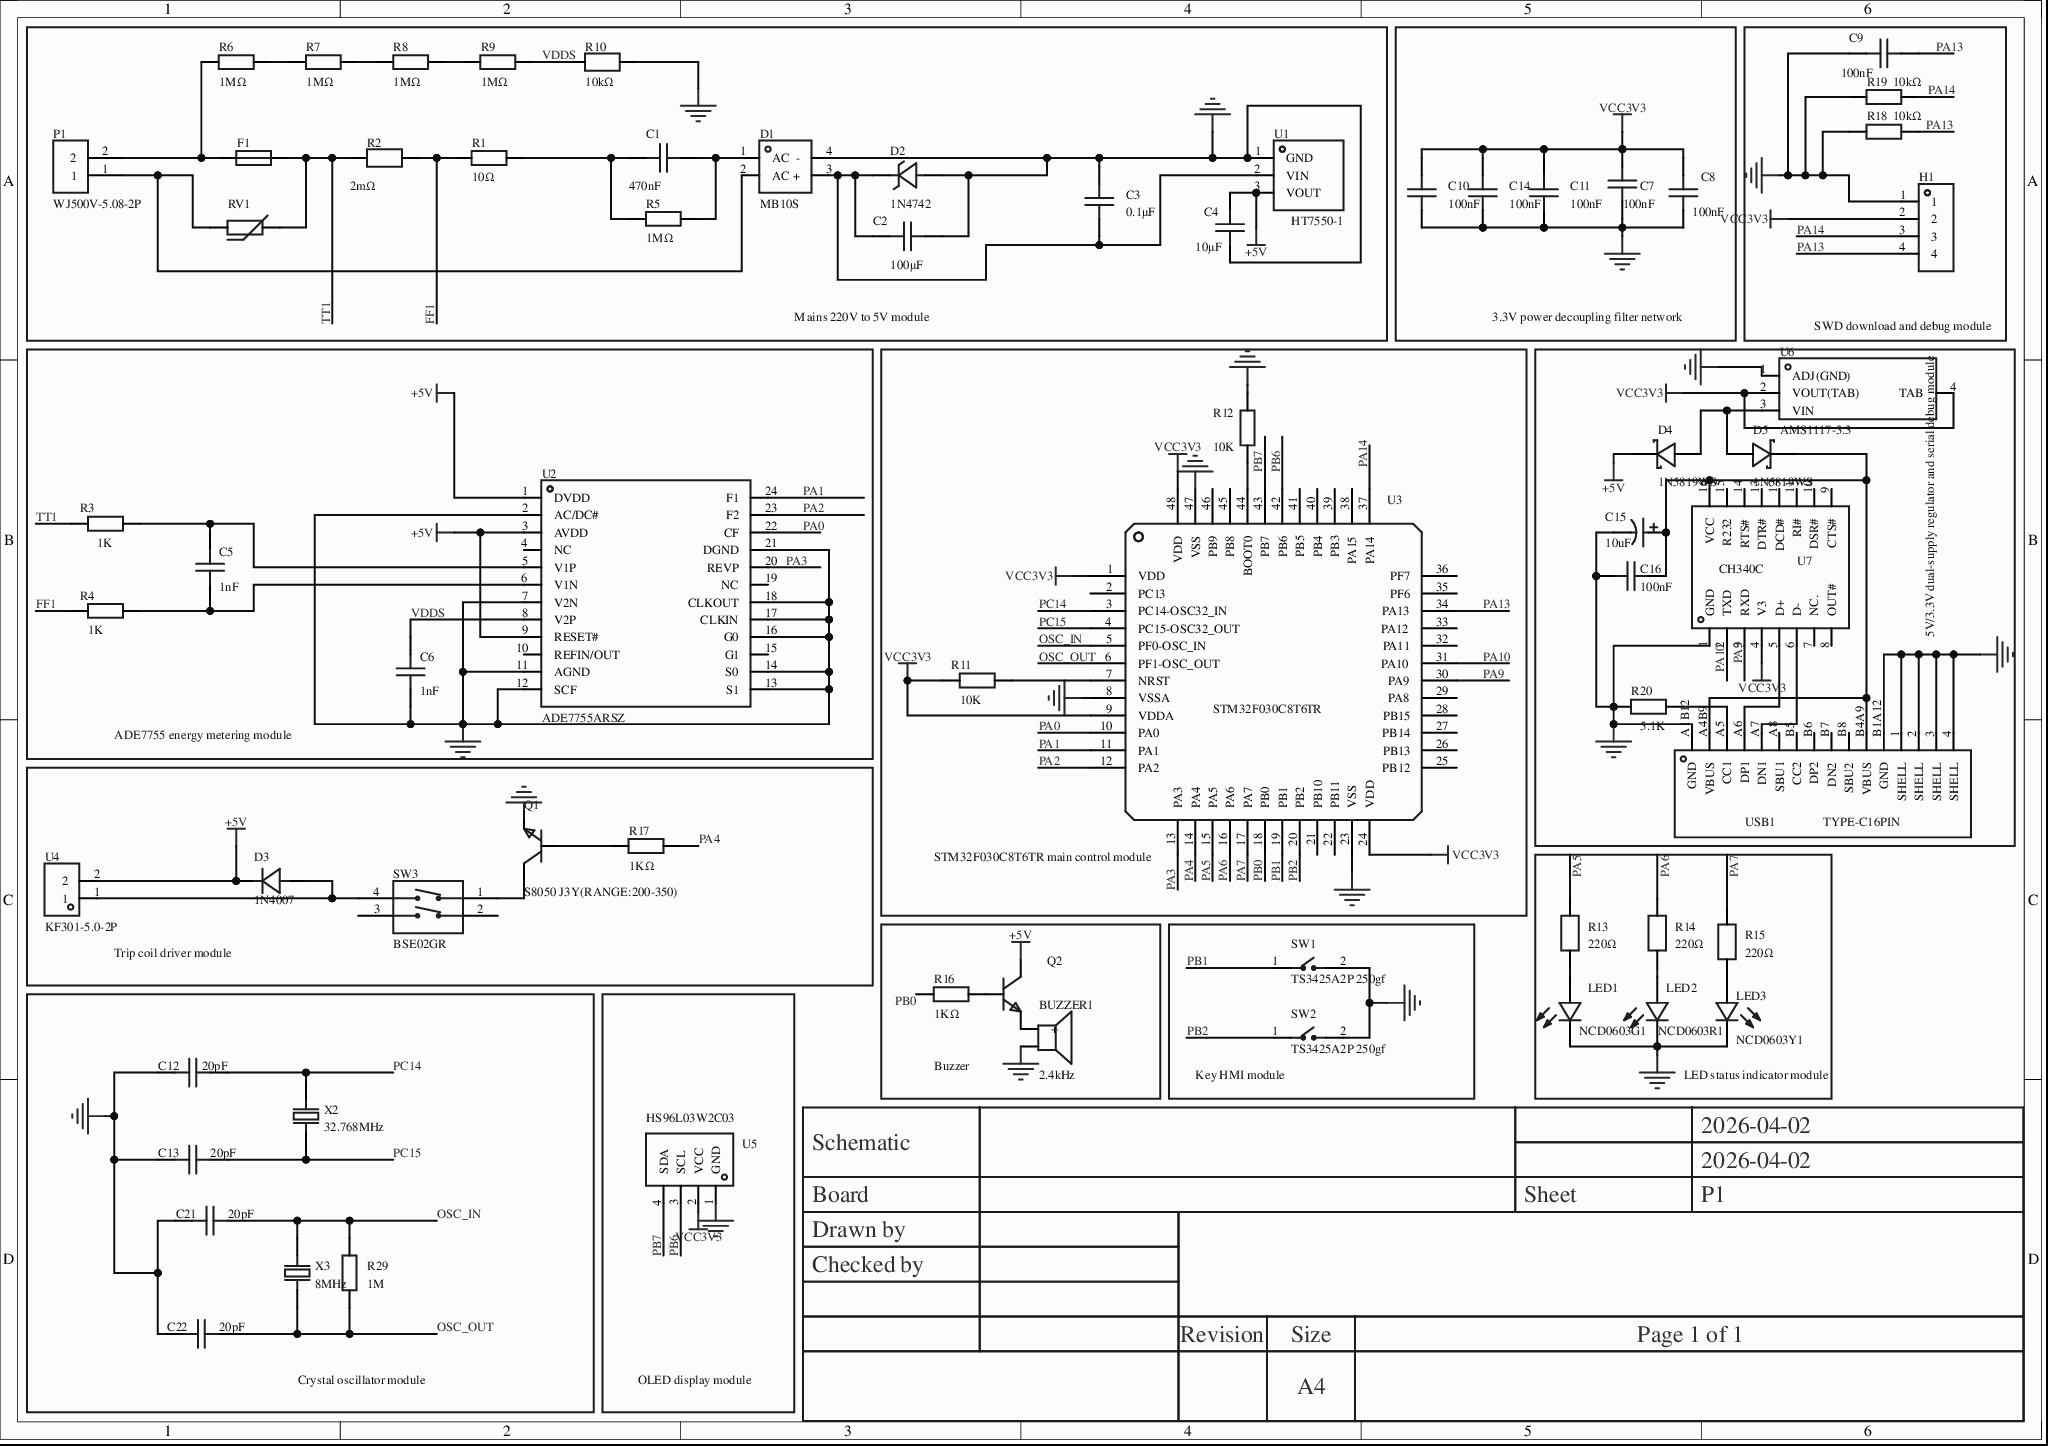
[diagram p0: MISC49877-3.schdoc]
# Altium project MISC49877-2.PrjPcb
1 sheet, 67 parts. Net scope: global (net labels, ports and power ports of the same name join across sheets).
Board file: MISC49877.pcbdoc

## Sheet MISC49877-3.schdoc
size 297 x 209 mm; Version: V1.0; @Project Name: MISC49877; @Update Date: 2026-04-09; @Create Date: 2026-04-09; @Board Name: MISC49877; @Create Time: 14:55:17; @Page Count: 1; @Page No: 1; @Schematic Name: MISC49877; @Update Time: 14:55:17; Size: A4

### Parts
BUZZER1  2.4kHz  [BUZ-TH_BD12.0-P7.60-D0.6-FD]
C1  470nF  [CAP-TH_L17.0-W5.5-P15.00-D1.2]
C2  100μF  [C0603]
C3  0.1μF  [C0603]
C4  10μF  [C0603]
C5  1nF  [C0603]
C6  1nF  [C0603]
C7  100nF  [C0805]
C8  100nF  [C0805]
C9  100nF  [C0603]
C10  100nF  [C0805]
C11  100nF  [C0603]
C12  20pF  [C0805]
C13  20pF  [C0805]
C14  100nF  [C0805]
C15  10uF  [CAP-SMD_BD5.0-L5.3-W5.3-FD]
C16  100nF  [C0603]
C21  20pF  [C0805]
C22  20pF  [C0805]
D1  MB10S  [MBS_L4.7-W4.0-P2.50-LS7.0-TL]
D2  1N4742  [DO-41_BD2.4-L4.7-P8.70-D0.8-FD]
D3  1N4007  [SMA_L4.3-W2.5-LS5.0-RD]
D4  1N5819WS  [SOD-323_L1.8-W1.3-LS2.5-RD]
D5  1N5819WS  [SOD-323_L1.8-W1.3-LS2.5-RD]
F1  2F.0500212000S1B02  [FUSE-TH_BD3.0-L7.2-P11.20-D0.6]  (value not drawn)
H1  (no value)  [HDR-TH_4P-P2.54-V-F]
LED1  NCD0603G1  [LED0603-RD_1]
LED2  NCD0603R1  [LED0603-RD_RED]
LED3  NCD0603Y1  [LED0603-RD]
P1  WJ500V-5.08-2P  [CONN-TH_2P-P5.00_WJ500V-5.08-2P]
Q1  S8050 J3Y(RANGE:200-350)  [SOT-23-3_L3.0-W1.7-P0.95-LS2.9-BR]
Q2  (no value)  [S8050_SOT-23]
R1  10Ω  [R0603]
R2  2mΩ  [RES-SMD_L6.4-W3.2-1]
R3  1K  [R0603]
R4  1K  [R0603]
R5  1MΩ  [R0603]
R6  1MΩ  [R1206]
R7  1MΩ  [R1206]
R8  1MΩ  [R1206]
R9  1MΩ  [R1206]
R10  10kΩ  [R0805]
R11  10K  [R0603]
R12  10K  [R0603]
R13  220Ω  [R0402]
R14  220Ω  [R0402]
R15  220Ω  [R0402]
R16  1KΩ  [R0603]
R17  1KΩ  [R0603]
R18  10kΩ  [R0805]
R19  10kΩ  [R0805]
R20  5.1K  [R0603]
R29  1M  [R0805]
RV1  190pF@1kHz  [RES-TH_L12.5-W6.7-P7.50-D1.2]  (value not drawn)
SW1  TS3425A2P 250gf  [SW-SMD_L3.9-W2.9-LS5.0]
SW2  TS3425A2P 250gf  [SW-SMD_L3.9-W2.9-LS5.0]
SW3  BSE02GR  [SW-TH_4P-L9.9-W6.8-P7.62-BL]
U1  HT7550-1  [SOT-89_L4.5-W2.5-P1.50-LS4.2-BR]
U2  ADE7755ARSZ  [SSOP-24_L8.1-W5.3-P0.65-LS7.8-BL]
U3  STM32F030C8T6TR  [LQFP-48_L7.0-W7.0-P0.50-LS9.0-BL]
U4  KF301-5.0-2P  [HDR-M-2.54_1X2]
U5  HS96L03W2C03  [OLED-TH_L27.8-W27.2-P2.54_C9900033791]
U6  AMS1117-3.3  [SOT-223-4_L6.5-W3.5-P2.30-LS7.0-BR]
U7  CH340C  [SOP-16_L10.0-W3.9-P1.27-LS6.0-BL]
USB1  TYPE-C16PIN  [USB-C-SMD_TYPE-C16PIN]
X2  32.768MHz  [CRYSTAL-SMD_L3.2-W2.5_3225-8MHZ]
X3  8MHz  [CRYSTAL-SMD_L3.2-W2.5_3225-8MHZ]

### Blocks framed on the sheet
Mains 220V to 5V module: C1-C4 D1 D2 F1 P1 R1 R2 R5-R10 RV1 U1
3.3V power decoupling filter network: C7 C8 C10 C11 C14
SWD download and debug module: C9 H1 R18 R19
ADE7755 energy metering module: C5 C6 R3 R4 U2
STM32F030C8T6TR main control module: R11 R12 U3
5V/3.3V dual-supply regulator and serial debug module: C15 C16 D4 D5 R20 U6 U7 USB1
Trip coil driver module: D3 Q1 R17 SW3 U4
LED status indicator module: LED1-LED3 R13-R15
Buzzer: BUZZER1 Q2 R16
Key HMI module: SW1 SW2
Crystal oscillator module: C12 C13 C21 C22 R29 X2 X3
OLED display module: U5

### Nets
+5V: C4.2 D3.1(K) D4.1(K) Q2.3 U1.3(VOUT) U2.1(DVDD) U2.3(AVDD) U2.9(RESET#) U4.2
GND: BUZZER1.2 C2.1 C3.2 C4.1 C6.1 C7.2 C8.1 C9.1 C10.2 C11.1 C12.2 C13.1 C14.1 C15.2 C16.1 C21.1 C22.1 D1.4(-) D2.1(A) H1.1 LED1.1(K) LED2.1(K) LED3.1(K) Q1.2(E) R10.2 R12.2 R18.2 R19.2 R20.2 SW1.2 SW2.2 U1.1(GND) U2.2(AC/DC#) U2.7(V2N) U2.11(AGND) U2.12(SCF) U2.13(S1) U2.14(S0) U2.16(G0) U2.17(CLKIN) U2.18(CLKOUT) U2.21(DGND) U3.8(VSSA) U3.23(VSS) U3.47(VSS) U5.1(GND) U6.1(ADJ(GND)) U7.1(GND) USB1.1(SHELL) USB1.2(SHELL) USB1.3(SHELL) USB1.4(SHELL) USB1.A1B12(GND) USB1.B1A12(GND)
VCC3V3: C7.1 C8.2 C10.1 C11.2 C14.2 H1.2 R11.1 U3.1(VDD) U3.9(VDDA) U3.24(VDD) U3.48(VDD) U5.2(VCC) U6.2(VOUT(TAB)) U6.4(TAB) U7.4(V3)
FF1: R1.1 R2.2 R4.1
OSC_IN: C21.2 R29.2 U3.5(PF0-OSC_IN) X3.2
OSC_OUT: C22.2 R29.1 U3.6(PF1-OSC_OUT) X3.1
PA0: U2.22(CF) U3.10(PA0)
PA1: U2.24(F1) U3.11(PA1)
PA2: U2.23(F2) U3.12(PA2)
PA3: U2.20(REVP) U3.13(PA3)
PA4: R17.1 U3.14(PA4)
PA5: R13.2 U3.15(PA5)
PA6: R14.2 U3.16(PA6)
PA7: R15.2 U3.17(PA7)
PA9: U3.30(PA9) U7.3(RXD)
PA10: U3.31(PA10) U7.2(TXD)
PA13: C9.2 H1.4 R18.1 U3.34(PA13)
PA14: H1.3 R19.1 U3.37(PA14)
PB0: R16.2 U3.18(PB0)
PB1: SW1.1 U3.19(PB1)
PB2: SW2.1 U3.20(PB2)
PB6: U3.42(PB6) U5.3(SCL)
PB7: U3.43(PB7) U5.4(SDA)
PC14: C12.1 U3.3(PC14-OSC32_IN) X2.2
PC15: C13.2 U3.4(PC15-OSC32_OUT) X2.1
TT1: F1.2 R2.1 R3.1 RV1.2
VDDS: C6.2 R9.2 R10.1 U2.8(V2P)
NetBUZZER1_1: BUZZER1.1(+) Q2.2
NetC1_1: C1.1 D1.1(AC) R5.2
NetC1_2: C1.2 R1.2 R5.1
NetC2_2: C2.2 C3.1 D1.3(+) D2.2(K) U1.2(VIN)
NetC5_1: C5.1 R4.2 U2.6(V1N)
NetC5_2: C5.2 R3.2 U2.5(V1P)
NetC15_1: C15.1 C16.2 D5.1(K) U7.16(VCC) USB1.A4B9(VBUS) USB1.B4A9(VBUS)
NetD1_2: D1.2(AC) P1.1 RV1.1
NetD3_2: D3.2(A) SW3.4 U4.1
NetD4_2: D4.2(A) D5.2(A) U6.3(VIN)
NetF1_1: F1.1 P1.2 R6.1
NetLED1_2: LED1.2(A) R13.1
NetLED2_2: LED2.2(A) R14.1
NetLED3_2: LED3.2(A) R15.1
NetQ1_1: Q1.1(B) R17.2
NetQ1_3: Q1.3(C) SW3.1
NetQ2_1: Q2.1 R16.1
NetR6_2: R6.2 R7.1
NetR7_2: R7.2 R8.1
NetR8_2: R8.2 R9.1
NetR11_2: R11.2 U3.7(NRST)
NetR12_1: R12.1 U3.44(BOOT0)
NetR20_1: R20.1 USB1.A5(CC1)
NetU7_5: U7.5(D+) USB1.A6(DP1)
NetU7_6: U7.6(D-) USB1.A7(DN1)

Not connected (* = marked no-connect by the designer): SW3 2* 3*; U2 4(NC)* 10(REFIN/OUT)* 15(G1)* 19(NC)*; U3 2(PC13)* 21(PB10)* 22(PB11)* 25(PB12)* 26(PB13)* 27(PB14)* 28(PB15)* 29(PA8)* 32(PA11)* 33(PA12)* 35(PF6)* 36(PF7)* 38(PA15)* 39(PB3)* 40(PB4)* 41(PB5)* 45(PB8)* 46(PB9)*; U7 7(NC.)* 8(OUT#)* 9(CTS#)* 10(DSR#)* 11(RI#)* 12(DCD#)* 13(DTR#)* 14(RTS#)* 15(R232)*; USB1 A8(SBU1)* B5(CC2)* B6(DP2)* B7(DN2)* B8(SBU2)*

### Notes on the sheet
- 2026-04-02
- Schematic
- Board
- Sheet
- P1
- Drawn by
- Checked by
- Revision
- Size
- A4
- Page 1 of 1

### Library data of the parts
BUZZER1 = TMB12A05_C96093: Drive method: active (built-in driver circuit); Construction type: electromagnetic; Rated voltage: 5V; Frequency: 2.4kHz; Sound pressure (SPL): 85dB;; Manufacturer: 华能; Voltage - Supply: 4V~8V; Current Consumption: 30mA; 3D Model: 16ab50e14c5b4f2c986c135bdba60e370819f05c4eef4c71ace90d822a990e87; 3D Model Transform: 472.44,472.176,0,90,0,0,-0.787,0,-177.165; AddInBom: yes; ModelName: BUZ-TH_D12.0-H9.5-P7.60; Device: TMB12A05_C96093; Symbol: TMB12A05; LCSC Part Name: 有源(内含驱动线路) 电磁式 2.4kHz; Supplier Part: C96093; Manufacturer Part: TMB12A05; Supplier Footprint: 插件,D=12mm; JLCPCB Part Class: Extended Part; Datasheet: https://item.szlcsc.com/datasheet/TMB12A05/97297.html; Supplier: LCSC; Driver Circuitry: Active (built-in driver circuit); Technology: Electromagnetic; Voltage Rating: 5V; Value: 2.4kHz; Sound Pressure Level(SPL): 85dB; Diameter(φD): 12mm; Length: -; Width: -; Height: 9.8mm; Operating Temperature: -40℃~+85℃; FootprintName: BUZ-TH_BD12.0-P7.60-D0.6-FD; ConvertToPcb: yes
C1 = CBB21-400V474JP15: Capacitance: 470nF; Tolerance: ±5%; Rated voltage: 400V; Operating temperature: -40℃~+105℃;; Manufacturer: 东通电子; AddInBom: yes; ModelId: f8cf251704e9467493657d330e769cf70819f05c4eef4c71ace90d822a990e87; ModelName: CAP-TH_L17.0-W5.5-H10.0-P15.0; ModelTransform: 669.29,216.535,0,0,0,0,0,0,-137.795; Device: CBB21-400V474JP15; Symbol: CBB21-400V474JP15; FootprintName: CAP-TH_L17.0-W5.5-P15.00-D1.2; LCSC Part Name: 470nF ±5% 400V; SupplierPart: C2888194; ManufacturerPart: CBB21-400V474JP15; Supplier Footprint: 插件,P=15mm; JLCPCB Part Class: Extended Part; Datasheet: https://item.szlcsc.com/datasheet/CBB21-400V474JP15/3107607.html; Supplier: LCSC; ConvertToPcb: yes; Value: 470nF; Voltage Rating: 400V; Operating Temperature: -40℃~+105℃
C2 = CAP_0603: Symbol: Capacitance; ConvertToPcb: yes; ModelId: ac125912035d415993ca9572d50418b10819f05c4eef4c71ace90d822a990e87; ModelName: C0603_L1.6-W0.8-H0.8; ModelTransform: 62.992,31.496,0,0,0,0,0,0,0; Device: CAP_0603; Value: 100μF; FootprintName: C0603; AddInBom: yes; Supplier Footprint: 0603
C3-C6 C11 = CAP_0603: Symbol: Capacitance; 3D Model: ac125912035d415993ca9572d50418b10819f05c4eef4c71ace90d822a990e87; 3D Model Transform: 62.992,31.496,0,0,0,0,0,0,0; ConvertToPcb: yes; ModelName: C0603_L1.6-W0.8-H0.8; Device: CAP_0603; Supplier Footprint: 0603; FootprintName: C0603; AddInBom: yes
  C3: Value: 0.1μF
  C4: Value: 10μF
  C5 C6: Value: 1nF
  C11: Value: 100nF
C7 C10 = GRM21BR71H104KA01L: Capacitance: 100nF; Tolerance: ±10%; Rated voltage: 50V; Temperature coefficient: X7R;; Manufacturer: muRata(村田); AddInBom: yes; ModelId: 1ba041120af144c991958decab20d2410819f05c4eef4c71ace90d822a990e87; ModelName: C0805_L2.0-W1.3-H1.3; ModelTransform: 78.74,51.181,0,0,0,0,0,0.0005,0; Device: GRM21BR71H104KA01L; Symbol: GRM21BR71H104KA01L; FootprintName: C0805; LCSC Part Name: 100nF ±10% 50V; SupplierPart: C77082; ManufacturerPart: GRM21BR71H104KA01L; Supplier Footprint: 0805; JLCPCB Part Class: Extended Part; Datasheet: https://item.szlcsc.com/datasheet/GRM21BR71H104KA01L/78209.html; Supplier: LCSC; ConvertToPcb: yes; Value: 100nF; Voltage Rating: 50V; Temperature Coefficient: X7R
C8 C14 = GRM21BR71H104KA01L: Capacitance: 100nF; Tolerance: ±10%; Rated voltage: 50V; Temperature coefficient: X7R;; Manufacturer: muRata(村田); 3D Model: 1ba041120af144c991958decab20d2410819f05c4eef4c71ace90d822a990e87; 3D Model Transform: 78.74,51.181,0,0,0,0,0,0.0005,0; AddInBom: yes; ModelName: C0805_L2.0-W1.3-H1.3; Device: GRM21BR71H104KA01L; Symbol: GRM21BR71H104KA01L; LCSC Part Name: 100nF ±10% 50V; Supplier Part: C77082; Manufacturer Part: GRM21BR71H104KA01L; Supplier Footprint: 0805; JLCPCB Part Class: Extended Part; Datasheet: https://item.szlcsc.com/datasheet/GRM21BR71H104KA01L/78209.html; Supplier: LCSC; Value: 100nF; Voltage Rating: 50V; Temperature Coefficient: X7R; FootprintName: C0805; ConvertToPcb: yes
C9 = FCC0603B104K500CT: Capacitance: 100nF; Tolerance: ±10%; Rated voltage: 50V; Temperature coefficient: X7R;; Manufacturer: FOJAN(富捷); AddInBom: yes; ModelId: ac125912035d415993ca9572d50418b10819f05c4eef4c71ace90d822a990e87; ModelName: C0603_L1.6-W0.8-H0.8; ModelTransform: 62.992,31.496,0,0,0,0,0,0,0; Device: FCC0603B104K500CT; Symbol: FCC0603B104K500CT; FootprintName: C0603; LCSC Part Name: 100nF ±10% 50V; SupplierPart: C5137636; ManufacturerPart: FCC0603B104K500CT; Supplier Footprint: 0603; JLCPCB Part Class: Extended Part; Datasheet: https://item.szlcsc.com/datasheet/FCC0603B104K500CT/5747088.html; Supplier: LCSC; ConvertToPcb: yes; Value: 100nF; Voltage Rating: 50V; Temperature Coefficient: X7R
C12 C13 C21 C22 = CAP_0805: Symbol: CapAcitance; 3D Model: 1ba041120af144c991958decab20d241; 3D Model Transform: 78.74,51.181,0,0,0,0,0,0.0005,0; ConvertToPcb: yes; ModelName: C0805_L2.0-W1.3-H1.3; Device: CAP_0805; Value: 20pF; Supplier Footprint: 0805; FootprintName: C0805; AddInBom: yes
C15 = RVT1H100M0505_C72487: Capacitance: 10uF; Tolerance: ±20%; Rated voltage: 50V; Ripple current: 17mA@120Hz; Equivalent series resistance (ESR): -;; Manufacturer: ROQANG(容强); AddInBom: yes; Lifetime: 2000hrs@105℃; ModelId: 16f5696d655347d6a4362817d02ce59a0819f05c4eef4c71ace90d822a990e87; ModelName: CAP-SMD_BD5.0-L5.3-W5.3-LS5.5-FD; ModelTransform: 216.535,208.661,0,0,0,0,0,0,0; Device: RVT1H100M0505_C72487; Symbol: RVT1H100M0505; FootprintName: CAP-SMD_BD5.0-L5.3-W5.3-FD; LCSC Part Name: 10uF ±20% 50V; SupplierPart: C72487; ManufacturerPart: RVT1H100M0505; Supplier Footprint: SMD,D5xL5.4mm; JLCPCB Part Class: Extended Part; Datasheet: https://item.szlcsc.com/datasheet/RVT1H100M0505/73598.html; Supplier: LCSC; ConvertToPcb: yes; Value: 10uF; Voltage Rating: 50V; Ripple Current: 17mA@120Hz; Equivalent Series Resistance(ESR): -; Diameter: 5mm; Height - Seated (Max): 5.4mm; Operating Temperature: -40℃~+105℃
C16 = CGA0603X7R104K500JT: Capacitance: 100nF; Tolerance: ±10%; Rated voltage: 50V; Temperature coefficient: X7R;; Manufacturer: HRE(芯声); AddInBom: yes; ModelId: ac125912035d415993ca9572d50418b10819f05c4eef4c71ace90d822a990e87; ModelName: C0603_L1.6-W0.8-H0.8; ModelTransform: 62.992,31.496,0,0,0,0,0,0,0; Device: CGA0603X7R104K500JT; Symbol: CGA0603X7R104K500JT; FootprintName: C0603; LCSC Part Name: 100nF ±10% 50V; SupplierPart: C6119867; ManufacturerPart: CGA0603X7R104K500JT; Supplier Footprint: 0603; JLCPCB Part Class: Extended Part; Datasheet: https://item.szlcsc.com/datasheet/CGA0603X7R104K500JT/7062573.html; Supplier: LCSC; ConvertToPcb: yes; Value: 100nF; Voltage Rating: 50V; Temperature Coefficient: X7R
D1 = MB10S_C42463381: Forward voltage (Vf): 1.1V@1A; DC reverse withstand voltage (Vr): 1kV; Rectified current: 1A; Non-repetitive peak surge current (Ifsm): 35A;; Manufacturer: R+O(宏嘉诚); AddInBom: yes; Reverse Leakage Current (Ir): 5uA; Operating Junction Temperature Range: -55℃~+150℃; ModelId: 7dad5ddbf7424b73bca0092e0c7e32040819f05c4eef4c71ace90d822a990e87; ModelName: MBS_L4.7-W4.0-H2.5-LS7.0; ModelTransform: 185.039,275.591,0,270,0,0,0,0,0; Device: MB10S_C42463381; Symbol: MB10S_C42463381; FootprintName: MBS_L4.7-W4.0-P2.50-LS7.0-TL; LCSC Part Name: 耐压:1000V 电流:1A; SupplierPart: C42463381; ManufacturerPart: MB10S; Supplier Footprint: MBS; JLCPCB Part Class: Extended Part; Datasheet: https://item.szlcsc.com/datasheet/MB10S/44554700.html; Supplier: LCSC; ConvertToPcb: yes; Voltage - Forward(Vf@If): 1.1V@1A; Voltage - DC Reverse(Vr): 1kV; Current - Rectified: 1A; Non-Repetitive Peak Forward Surge Current: 35A
D2 = 1N4742: Diode configuration: standalone; Zener voltage (nominal): 12V; Zener voltage (range): 11.45V~12.95V; Power dissipation (Pd): 1W;; Manufacturer: LGE(鲁光); AddInBom: yes; Reverse Leakage Current (Ir): 5uA; Impedance(Zzt): 9Ω; Impedance(Zzk): 700Ω; ModelId: 6de1e9b71a0d4751b4e9df530304c1a30819f05c4eef4c71ace90d822a990e87; ModelName: DO-41_D2.4-L4.7-P8.70; ModelTransform: 374.015,94.428,0,180,0,0,0,0,-137.795; Device: 1N4742; Symbol: 1N4742; FootprintName: DO-41_BD2.4-L4.7-P8.70-D0.8-FD; LCSC Part Name: 独立式 耐压:12V 电流:5uA; SupplierPart: C5174492; ManufacturerPart: 1N4742; Supplier Footprint: DO-41; JLCPCB Part Class: Extended Part; Datasheet: https://item.szlcsc.com/datasheet/1N4742/5826851.html; Supplier: LCSC; ConvertToPcb: yes; Diode Configuration: Standalone; Zener Voltage(Nom): 12V; Zener Voltage(Range): 11.45V~12.95V; Pd - Power Dissipation: 1W
D3 = 1N4007_C727081: Diode configuration: standalone; Forward voltage (Vf): 1.1V@1A; DC reverse withstand voltage (Vr): 1kV; Rectified current: 1A;; Manufacturer: TWGMC(迪嘉); AddInBom: yes; Reverse Leakage Current (Ir): 5uA; ModelId: 5b53cc1b87a148cc9fa13125be89f9480819f05c4eef4c71ace90d822a990e87; ModelTransform: 194.8815,98.425,0,0,0,0,0,0,0; Device: 1N4007_C727081; Symbol: 1N4007_C727081; FootprintName: SMA_L4.3-W2.5-LS5.0-RD; LCSC Part Name: 1N4007; SupplierPart: C727081; ManufacturerPart: 1N4007; Supplier Footprint: SMA(DO-214AC); JLCPCB Part Class: Extended Part; Datasheet: https://item.szlcsc.com/datasheet/1N4007/774186.html; Supplier: LCSC; ConvertToPcb: yes; Diode Configuration: Standalone; Voltage - Forward(Vf@If): 1.1V@1A; Voltage - DC Reverse(Vr): 1kV; Current - Rectified: 1A; ModelName: SMA_L4.3-W2.5-LS5.0-RD
D4 D5 = 1N5819WS_C191023: Forward voltage (Vf): 600mV@1A; DC reverse withstand voltage (Vr): 40V; Rectified current: 1A;; Manufacturer: Hottech(合科泰); AddInBom: yes; ModelId: db63db13d9e342eb939127d413d6200b0819f05c4eef4c71ace90d822a990e87; ModelTransform: 104.3305,51.181,0,0,0,0,0,0,0; Non-Repetitive Peak Forward Surge Current: 25A; Symbol: 1N5819WS; Device: 1N5819WS_C191023; LCSC Part Name: 电压:40V 电流:1A; SupplierPart: C191023; ManufacturerPart: 1N5819WS; Supplier Footprint: SOD-323; JLCPCB Part Class: Basic Part; Datasheet: https://item.szlcsc.com/datasheet/1N5819WS/213850.html; Supplier: LCSC; ConvertToPcb: yes; FootprintName: SOD-323_L1.8-W1.3-LS2.5-RD; ModelName: SOD-323_L1.8-W1.3-LS2.5-RD; Voltage - Forward(Vf@If): 600mV@1A; Voltage - DC Reverse(Vr): 40V; Current - Rectified: 1A
F1 = 2F.0500212000S1B02: Type: glass tube fuse; Rated current: 500mA; Rated voltage (AC): 250V；125V; Breaking capacity: 50A;; Manufacturer: xcfuse(旭程); Symbol: 2F500MA 250V; AddInBom: yes; Voltage Rating (AC): 250V; 125V; Melting I2t: 0.1; ModelId: 8493180d87ef424b8637a2753ca991c60819f05c4eef4c71ace90d822a990e87; ModelName: FUSE-TH_BD3.4-L7.1-P11.20-D0.6; ModelTransform: 497.6368,134.6891,0,0,0,0,0,0,-196.85; Device: 2F.0500212000S1B02; FootprintName: FUSE-TH_BD3.0-L7.2-P11.20-D0.6; LCSC Part Name: 插件式保险丝; SupplierPart: C140536; ManufacturerPart: 2F.0500212000S1B02; Supplier Footprint: 插件,D2.7xL7.3mm; JLCPCB Part Class: Extended Part; Datasheet: https://item.szlcsc.com/datasheet/2F.0500212000S1B02/151862.html; Supplier: LCSC; ConvertToPcb: yes; Type: Glass tube fuse; Current Rating: 500mA; Operating Temperature: -40℃~+125℃; Interrupt Rating: 50A; Diameter (φD): 2.7mm; Length: 7.3mm
H1 = HDR-F_2.54_1x4P: Symbol: 2.54-1*4P female; ConvertToPcb: yes; ModelId: d187812051054f85879fcaa51a310d8e0819f05c4eef4c71ace90d822a990e87; ModelTransform: 419.6842,98.464,0,0,0,0,0,0,-118.11; Device: HDR-F_2.54_1x4P; AddInBom: yes; SupplierPart: C2718488; Supplier Footprint: 插件; FootprintName: HDR-TH_4P-P2.54-V-F; ModelName: HDR-TH_4P-P2.54-V-F
LED1 = NCD0603G1: Lamp type: -; Light colour: emerald green; Forward voltage (Vf): 2.6V~3.6V; Power: 72mW; Forward current: 20mA; Wavelength: 515nm~530nm; Diode configuration: standalone diode; Lens colour: -; Colour temperature: -; Luminous intensity: 900mcd; Viewing angle: 130°; Packaging: -; Operating temperature: -30℃~+85℃;; Manufacturer: 国星光电; Symbol: FC-D1608UGK-520D10; Add into BOM: yes; 3D Model: 3beb0148d24d477aac1d9f7d4b6d534c; 3D Model Transform: 62.2046,31.496,0,0,0,0,-1.948,0.215,0; Peak Wavelength: 520nm; Device: NCD0603G1; Convert to PCB: yes; LCSC Part Name: 片式发光二极管; Supplier Part: C84267; Manufacturer Part: NCD0603G1; Supplier Footprint: 0603; JLCPCB Part Class: Extended Part; Datasheet: https://item.szlcsc.com/datasheet/NCD0603G1/85436.html; Supplier: LCSC; Lamp Holder Type: -; Illumination Color: Emerald green; Voltage - Forward(Vf): 2.6V~3.6V; Power(Watts): 72mW; Forward Current: 20mA; Wavelength - Dominant: 515nm~530nm; Diode Configuration: Standalone diode; Lens Color: -; Color Temperature: -; Luminous Intensity: 900mcd; Viewing Angle: 130°; Mounting Style: -; Operating Temperature: -30℃~+85℃; FootprintName: LED0603-RD_1; ModelName: LED0603-RD_1
LED2 = NCD0603R1_C84263: Lamp type: -; Light colour: red; Forward voltage (Vf): 1.6V~2.6V; Power: 65mW; Forward current: 25mA; Wavelength: 615nm~630nm; Diode configuration: standalone diode; Lens colour: -; Colour temperature: -; Luminous intensity: 220mcd; Viewing angle: 130°; Packaging: -; Operating temperature: -30℃~+85℃;; Manufacturer: 国星光电; Symbol: FC-DA1608HRK-620D; AddInBom: yes; Peak Wavelength: 630nm; ModelId: 74041d3a270d435c8600a9ab9b7641c00819f05c4eef4c71ace90d822a990e87; ModelTransform: 63.7794,31.496,0,0,0,0,0,-0.002,0; Device: NCD0603R1_C84263; FootprintName: LED0603-RD_RED; LCSC Part Name: 片式发光二极管; SupplierPart: C84263; ManufacturerPart: NCD0603R1; Supplier Footprint: 0603; JLCPCB Part Class: Extended Part; Datasheet: https://item.szlcsc.com/datasheet/NCD0603R1/85432.html; Supplier: LCSC; ConvertToPcb: yes; Lamp Holder Type: -; Illumination Color: Red; Voltage - Forward(Vf): 1.6V~2.6V; Power(Watts): 65mW; Forward Current: 25mA; Wavelength - Dominant: 615nm~630nm; Diode Configuration: Standalone diode; Lens Color: -; Color Temperature: -; Luminous Intensity: 220mcd; Viewing Angle: 130°; Mounting Style: -; Operating Temperature: -30℃~+85℃; ModelName: LED0603-RD_RED
LED3 = NCD0603Y1: Lamp type: -; Light colour: yellow; Forward voltage (Vf): 1.6V~2.6V; Power: 65mW; Forward current: 25mA; Wavelength: 586nm~595nm; Diode configuration: standalone diode; Lens colour: -; Colour temperature: -; Luminous intensity: 220mcd; Viewing angle: 130°; Packaging: -; Operating temperature: -30℃~+85℃;; Manufacturer: 国星光电; Symbol: FC-D1608HYK-588J; AddInBom: yes; Peak Wavelength: 595nm; ModelId: 1f0d29a91be547639d425604e9b96ebb0819f05c4eef4c71ace90d822a990e87; ModelTransform: 63.7794,32.283,0,0,0,0,0,0,0; Device: NCD0603Y1; FootprintName: LED0603-RD; LCSC Part Name: 片式发光二极管; SupplierPart: C84268; ManufacturerPart: NCD0603Y1; Supplier Footprint: 0603; JLCPCB Part Class: Extended Part; Datasheet: https://item.szlcsc.com/datasheet/NCD0603Y1/85437.html; Supplier: LCSC; ConvertToPcb: yes; Lamp Holder Type: -; Illumination Color: Yellow; Voltage - Forward(Vf): 1.6V~2.6V; Power(Watts): 65mW; Forward Current: 25mA; Wavelength - Dominant: 586nm~595nm; Diode Configuration: Standalone diode; Lens Color: -; Color Temperature: -; Luminous Intensity: 220mcd; Viewing Angle: 130°; Mounting Style: -; Operating Temperature: -30℃~+85℃; ModelName: LED0603-RD
P1 = WJ500V-5.08-2P: Structure: 1x2P; Pitch: 5.08mm; Colour: green; Mounting: through-hole; Rated current: 18A; Rated voltage: 250V; Rows: 1; Wire gauge - AWG: 14~30; Wire gauge - mm²: 2.5; Pins per row: 2; Contact material: -; Contact plating: -; Operating temperature range: -40℃~+105℃; Soldering temperature (max): -;; Manufacturer: KANGNEX(康奈克斯电气); Symbol: WJ500V-5.08-2P-14-00A; AddInBom: yes; Wire Gauge - mm2: 2.5; Number of PINs Per Row: 2; Screw Specification: M2.5; ModelId: 0f4a503c8d3b4ae19ed61267f5e9a1d70819f05c4eef4c71ace90d822a990e87; ModelTransform: 423.621,393.7,0,0,0,0,-11.811,19.685,-137.795; Device: WJ500V-5.08-2P; FootprintName: CONN-TH_2P-P5.00_WJ500V-5.08-2P; LCSC Part Name: 1x2P 5.08mm 直插 排数:1 每排P数:2; SupplierPart: C8465; ManufacturerPart: WJ500V-5.08-2P; Supplier Footprint: 插件,P=5.08mm; JLCPCB Part Class: Extended Part; Datasheet: https://atta.szlcsc.com/upload/public/pdf/source/20191225/C8465_02D34CE5B5B4A53DF5891601D97FA9F4.pdf; Supplier: LCSC; ConvertToPcb: yes; Color: Green; Mounting Style: Through-hole; Current Rating (Max): 18A; Voltage Rating (Max): 250V; Number of Pins: 2P; Number of Rows: 1; Wire Gauge - AWG: 14~30; Contact Material: -; Contact Plating: -; Operating Temperature Range: -40℃~+105℃; Soldering Temperature(Max): -; ModelName: CONN-TH_2P-P5.00_WJ500V-5.08-2P
Q1 = S8050 J3Y(RANGE:200-350): Transistor type: NPN; Collector current (Ic): 500mA; Collector-emitter breakdown voltage (Vceo): 25V; Power dissipation (Pd): 300mW; DC current gain (hFE): 200@500mA,1V;; Manufacturer: CJ(江苏长电/长晶); Symbol: S8050_C2146; AddInBom: yes; Transition frequency(fT): 150MHz; Current - Collector Cutoff: 100nA; Vce Saturation(VCE(sat)): 600mV@500mA,50mA; Emitter-Base Voltage(Vebo): 5V; Number: 1 NPN; ModelId: 89cb27a44ab2466697082bb9fd73a7d00819f05c4eef4c71ace90d822a990e87; ModelName: SOT-23-3L_L2.9-W1.6-H1.1-LS2.8-P0.95; ModelTransform: 114.173,110.236,0,90,0,0,0,0,0; Device: S8050 J3Y(RANGE:200-350); FootprintName: SOT-23-3_L3.0-W1.7-P0.95-LS2.9-BR; LCSC Part Name: H档(200-350) NPN 电流:0.5A 电压:25V; SupplierPart: C2146; ManufacturerPart: S8050 J3Y(RANGE:200-350); Supplier Footprint: SOT-23; JLCPCB Part Class: Basic Part; Datasheet: https://item.szlcsc.com/datasheet/S8050%2520J3Y(RANGE%253A200-350)/2503.html; Supplier: LCSC; ConvertToPcb: yes; type: NPN; Current - Collector(Ic): 500mA; Collector - Emitter Voltage VCEO: 25V; Pd - Power Dissipation: 300mW; DC Current Gain: 200@500mA,1V; Operating Temperature: -55℃~+150℃
Q2 = S8050_SOT_NPN: Symbol: NPN; ConvertToPcb: yes; ModelId: c62791f0466c4ae2a892c056b845b0ca0819f05c4eef4c71ace90d822a990e87; ModelName: SOT-23-3P_L2.9-W1.3-H1.0-LS2.4-P0.95; ModelTransform: 98.6,114.12,41.29,180,0,0,0,0,-3; Device: S8050_SOT_NPN; AddInBom: yes; Supplier Footprint: SOT-23; FootprintName: S8050_SOT-23
R1 R3-R5 R11 R12 R16 R17 = Res_0603: Symbol: Resistor; 3D Model: fc143cca1e79419f9cd78b61e9279f080819f05c4eef4c71ace90d822a990e87; 3D Model Transform: 31.8897,63.7794,0,90,0,0,0,0,0; ConvertToPcb: yes; Device: Res_0603; Supplier Footprint: 0603; FootprintName: R0603; AddInBom: yes; ModelName: R0603
  R1: Value: 10Ω
  R3 R4: Value: 1K
  R5: Value: 1MΩ
  R11 R12: Value: 10K
  R16 R17: Value: 1KΩ
R2 = HoLLR2512-3W-2mR-1%: Resistor type: sampling resistor; Resistance: 2mΩ; Tolerance: ±1%; Rated voltage drop: -; Power: 3W; Temperature coefficient: ±50ppm/℃; Mounting: SMD;; Manufacturer: Milliohm(毫欧); AddInBom: yes; Rated Current: 77.5A; ModelId: 2a92684014bd46c593e4aa7ce823c3500819f05c4eef4c71ace90d822a990e87; ModelTransform: 251.968,125.984,0,0,0,0,0,0,0; Device: HoLLR2512-3W-2mR-1%; Symbol: HOLLR2512-3W-2MR-1%; FootprintName: RES-SMD_L6.4-W3.2-1; LCSC Part Name: 2mΩ ±1% 3W; SupplierPart: C2994640; ManufacturerPart: HoLLR2512-3W-2mR-1%; Supplier Footprint: 2512; JLCPCB Part Class: Extended Part; Datasheet: https://atta.szlcsc.com/upload/public/pdf/source/20220330/9E8D3880B1628B3B70C68092C8A7E08B.pdf; Supplier: LCSC; ConvertToPcb: yes; Type: Sampling resistor; Value: 2mΩ; Rated Output Voltage: -; Power(Watts): 3W; Temperature Coefficient: ±50ppm/℃; Mounting Sytle: SMD; ModelName: RES-SMD_L6.4-W3.2-1
R6-R9 = 1206W4F1004T5E: Resistor type: thick film resistor; Resistance: 1MΩ; Tolerance: ±1%; Power: 250mW; Working voltage: 200V; Temperature coefficient: ±100ppm/℃;; Manufacturer: UNI-ROYAL(厚声); AddInBom: yes; ModelId: 89a1f13db2384da588040e0b3c55bf660819f05c4eef4c71ace90d822a990e87; ModelName: R1206_L3.2-W1.6-H0.6; ModelTransform: 125.984,62.992,0,0,0,0,0,0,0; Device: 1206W4F1004T5E; Symbol: 1206W4F1004T5E; FootprintName: R1206; LCSC Part Name: 1MΩ ±1% 250mW 厚膜电阻; SupplierPart: C17927; ManufacturerPart: 1206W4F1004T5E; Supplier Footprint: 1206; JLCPCB Part Class: Basic Part; Datasheet: https://item.szlcsc.com/datasheet/1206W4F1004T5E/18615.html; Supplier: LCSC; ConvertToPcb: yes; Type: Thick film resistor; Value: 1MΩ; Power(Watts): 250mW; Voltage-Supply(Max): 200V; Temperature Coefficient: ±100ppm/℃; Operating Temperature: -55℃~+155℃
R10 = RN73H2ATTD1002F50: Resistor type: metal film resistor; Resistance: 10kΩ; Tolerance: ±1%; Power: 125mW; Working voltage: -; Temperature coefficient: ±50ppm/℃;; Manufacturer: KOA; AddInBom: yes; ModelId: 37a81e68749a4138bd2dfa6897b24b850819f05c4eef4c71ace90d822a990e87; ModelName: R0805_L2.0-W1.3-H0.6; ModelTransform: 78.74,51.181,0,0,0,0,0,-0.0005,0; Device: RN73H2ATTD1002F50; Symbol: RN73H2ATTD1002F50; FootprintName: R0805; LCSC Part Name: 金属膜电阻 10kΩ ±1% 125mW; SupplierPart: C2519667; ManufacturerPart: RN73H2ATTD1002F50; Supplier Footprint: 0805; JLCPCB Part Class: Extended Part; Datasheet: https://atta.szlcsc.com/upload/public/pdf/source/20240329/18AD19F217F5EF2CC9094BC398D632CF.pdf; Supplier: LCSC; ConvertToPcb: yes; Type: Metal film resistor; Value: 10kΩ; Power(Watts): 125mW; Voltage-Supply(Max): -; Temperature Coefficient: ±50ppm/℃; Operating Temperature: -55℃~+155℃
R13-R15 = FRC0402F2200TS: Resistor type: thick film resistor; Resistance: 220Ω; Tolerance: ±1%; Power: 62.5mW; Working voltage: 50V; Temperature coefficient: ±100ppm/℃;; Manufacturer: FOJAN(富捷); AddInBom: yes; ModelId: 98c88bc2b9094f218f3a3e30a70127380819f05c4eef4c71ace90d822a990e87; ModelName: R0402_L1.0-W0.5-H0.4; ModelTransform: 39.37,19.685,0,0,0,0,0,0,0; Device: FRC0402F2200TS; Symbol: FRC0402F2200TS; FootprintName: R0402; LCSC Part Name: 220Ω ±1% 62.5mW 厚膜电阻; SupplierPart: C2909336; ManufacturerPart: FRC0402F2200TS; Supplier Footprint: 0402; JLCPCB Part Class: Extended Part; Datasheet: https://item.szlcsc.com/datasheet/FRC0402F2200TS/3186271.html; Supplier: LCSC; ConvertToPcb: yes; Type: Thick film resistor; Value: 220Ω; Power(Watts): 62.5mW; Voltage-Supply(Max): 50V; Temperature Coefficient: ±100ppm/℃; Operating Temperature: -55℃~+155℃
R18 R19 = 0805W8F1002T5E_C17414: Resistor type: thick film resistor; Resistance: 10kΩ; Tolerance: ±1%; Power: 125mW; Working voltage: 150V; Temperature coefficient: ±100ppm/℃;; Manufacturer: UNI-ROYAL(厚声); AddInBom: yes; ModelId: 37a81e68749a4138bd2dfa6897b24b850819f05c4eef4c71ace90d822a990e87; ModelName: R0805_L2.0-W1.3-H0.6; ModelTransform: 78.74,51.181,0,0,0,0,0,-0.0005,0; Device: 0805W8F1002T5E_C17414; Symbol: 0805W8F1002T5E; FootprintName: R0805; LCSC Part Name: 10kΩ ±1% 125mW 厚膜电阻; SupplierPart: C17414; ManufacturerPart: 0805W8F1002T5E; Supplier Footprint: 0805; JLCPCB Part Class: Basic Part; Datasheet: https://item.szlcsc.com/datasheet/0805W8F1002T5E/18102.html; Supplier: LCSC; ConvertToPcb: yes; Type: Thick film resistor; Value: 10kΩ; Power(Watts): 125mW; Voltage-Supply(Max): 150V; Temperature Coefficient: ±100ppm/℃; Operating Temperature: -55℃~+155℃
R20 = Res_0603: Symbol: Resistor; ConvertToPcb: yes; ModelId: fc143cca1e79419f9cd78b61e9279f080819f05c4eef4c71ace90d822a990e87; ModelTransform: 31.8897,63.7794,0,90,0,0,0,0,0; Device: Res_0603; Value: 5.1K; FootprintName: R0603; AddInBom: yes; Supplier Footprint: 0603; ModelName: R0603
R29 = Res_0805: Symbol: Resistor; 3D Model: 37a81e68749a4138bd2dfa6897b24b85; 3D Model Transform: 78.74,51.181,0,0,0,0,0,-0.0005,0; ConvertToPcb: yes; ModelName: R0805_L2.0-W1.3-H0.6; Device: Res_0805; Value: 1M; Supplier Footprint: 0805; FootprintName: R0805; AddInBom: yes
RV1 = 10D471K_C8760: Varistor voltage: 423V~517V; Clamping voltage: 775V; Working voltage (DC): 385V; Working voltage (AC): 300V;; Manufacturer: RUILON(瑞隆源); Symbol: 10D471K-C8760; AddInBom: yes; Peak Current: 2.5kA; Energy: 42.3J; Rated Wattage: 400mW; ModelId: fcca3f9494a74590ab8e2cf67301bbb60819f05c4eef4c71ace90d822a990e87; ModelName: RES-TH_L12.5-W6.7-P7.50-S6.3; ModelTransform: 492.075,271.653,0,0,0,0,0,0,-137.795; Device: 10D471K_C8760; FootprintName: RES-TH_L12.5-W6.7-P7.50-D1.2; LCSC Part Name: 钳位电压775V 42.3焦耳 插件压敏电阻; SupplierPart: C8760; ManufacturerPart: 10D471K; Supplier Footprint: 插件,P=7.5mm; JLCPCB Part Class: Extended Part; Datasheet: https://item.szlcsc.com/datasheet/10D471K/9271.html; Supplier: LCSC; ConvertToPcb: yes; Varistor Voltage: 423V~517V; Clamping Voltage: 775V; Maximum DC Volts: 385V; Maximum AC Volts: 300V; Value: 190pF@1kHz
SW1 SW2 = TS3425A2P 250gf: Circuit structure: SPST; Button shape: round button; Actuating force: 2.5N; Mounting: vertical SMD; Switch length: 3.9mm; Switch width: 2.9mm; Switch height: 2.5mm; Bracket: without bracket; Contact current: 50mA; Rated voltage: 12V; Lamp: none; Operating life: 5 ten-thousand cycles;; Manufacturer: SHOU HAN(首韩); AddInBom: yes; Actuator/Cap Color: Black; ModelId: 284ae12b719245d9ac94bed245e30d2a0819f05c4eef4c71ace90d822a990e87; ModelTransform: 196.85,114.173,0,0,0,0,0,0,0; Device: TS3425A2P 250gf; Symbol: TS3425A2P 250GF; FootprintName: SW-SMD_L3.9-W2.9-LS5.0; LCSC Part Name: 正按小龟 3*4*2.5mm 两脚不带柱 250gf; SupplierPart: C7431069; ManufacturerPart: TS3425A2P 250gf; Supplier Footprint: SMD; JLCPCB Part Class: Extended Part; Datasheet: https://item.szlcsc.com/datasheet/TS3425A2P%2520250gf/8431421.html; Supplier: LCSC; ConvertToPcb: yes; Circuit: SPST; Actuator Style: Round button; Operating Force: 2.5N; Mounting Type: Vertical SMD; Length: 3.9mm; Width: 2.9mm; Switch Height: 2.5mm; with Bracket: Without bracket; Contact Current: 50mA; Voltage Rating: 12V; With Lamp: None; Termination Style: SMD tabs; Life: 5 ten-thousand cycles; Operating Temperature: -20℃~+70℃; ModelName: SW-SMD_L3.9-W2.9-LS5.0
SW3 = BSE02GR: Circuit structure: SPST; Number of positions: 2; Rated current: 25mA; Rated voltage: 24V; Operating life: 2 thousand cycles; Colour: red;; Manufacturer: BIWIN(百莹); AddInBom: yes; Number of Positions: 2 positions; ModelId: 63ebfb56372a4ceba18c0aed18e1c9250819f05c4eef4c71ace90d822a990e87; ModelTransform: 259.881,389.763,0,0,0,0,0,0,-153.543; Device: BSE02GR; Symbol: BSE02GR; FootprintName: SW-TH_4P-L9.9-W6.8-P7.62-BL; LCSC Part Name: 2.54mm间距2P 红色插件拨码开关; SupplierPart: C3294681; ManufacturerPart: BSE02GR; Supplier Footprint: 插件,P=2.54mm; JLCPCB Part Class: Extended Part; Datasheet: https://item.szlcsc.com/datasheet/BSE02GR/3859081.html; Supplier: LCSC; ConvertToPcb: yes; Circuit: SPST; Termination Style: -; Lead Pitch: 2.54mm; Current Rating: 25mA; Voltage Rating: 24V; Operating Temperature: -40℃~+80℃; Operating Life: 2 thousand cycles; Color: Red; ModelName: SW-TH_4P-L9.9-W6.8-P7.62-BL
U1 = HT7550-1_C347189: Output type: fixed; Operating voltage: 30V; Output voltage: 5V; Output current: 100mA; PSRR: -; Output polarity: positive;; Manufacturer: UMW(友台半导体); 3D Model: 6db690b7897d4d18a30d90c1b89525ee0819f05c4eef4c71ace90d822a990e87; 3D Model Transform: 161.417,169.291,0,180,0,0,-12.745,0.006,0; Voltage Dropout: 100mV@(1mA); standby current: 3uA; Number of Outputs: 1; AddInBom: yes; ModelName: SOT-89-3_L4.3-W2.5-H1.6-LS4.1-P1.50; Device: HT7550-1_C347189; Symbol: HT7550-1_C347189; LCSC Part Name: 输入30V 输出5V 100mA; Supplier Part: C347189; Manufacturer Part: HT7550-1; Supplier Footprint: SOT-89; JLCPCB Part Class: Extended Part; Datasheet: https://item.szlcsc.com/datasheet/HT7550-1/323849.html; Supplier: LCSC; Output Type: Fixed; Voltage - Supply: 30V; Output Voltage: 5V; Output Current: 100mA; Power Supply Rejection Ratio (PSRR): -; Noise: -; Operating Temperature: -25℃~+70℃; Output Configuration: Positive; FootprintName: SOT-89_L4.5-W2.5-P1.50-LS4.2-BR; ConvertToPcb: yes
U2 = ADE7755ARSZ: Operating voltage: 4.75V~5.25V; Operating current: 3.5mA;; Manufacturer: ADI(亚德诺); 3D Model: f5b2473ce40e4151ba004f11ac5dda6c0819f05c4eef4c71ace90d822a990e87; 3D Model Transform: 322.834,307.086,0,0,0,0,0,0,0; Number of Channels: 2; Dynamic Range: 500:1; AddInBom: yes; ModelName: SSOP-24_L8.2-W5.3-H1.8-LS7.8-P0.65; Device: ADE7755ARSZ; Symbol: ADE7755ARSZ; LCSC Part Name: ADE7755 电能计量IC; Supplier Part: C1523825; Manufacturer Part: ADE7755ARSZ; Supplier Footprint: SSOP-24; JLCPCB Part Class: Extended Part; Datasheet: https://item.szlcsc.com/datasheet/ADE7755ARSZ/1614623.html; Supplier: LCSC; Voltage - Supply: 4.75V~5.25V; Current - Supply: 3.5mA; Operating Temperature: -40℃~+85℃; FootprintName: SSOP-24_L8.1-W5.3-P0.65-LS7.8-BL; ConvertToPcb: yes
U3 = STM32F030C8T6TR: CPU core: ARM-M0; Max CPU frequency: 48MHz; Application field: -;; Manufacturer: ST(意法半导体); AddInBom: yes; Program Storage Size: 64KB; Program Memory Type: FLASH; Number of I/O: 39; ADC (Bit): 12bit; Voltage - Supply: 2.4V~3.6V; ModelId: 093be70396ff421eb2cdb946d5311efc0819f05c4eef4c71ace90d822a990e87; ModelName: LQFP-48_L7.0-W7.0-H1.4-LS9.0-P0.50; ModelTransform: 354.331,354.331,0,0,0,0,0,0,0; Device: STM32F030C8T6TR; Symbol: STM32F030C8T6TR; FootprintName: LQFP-48_L7.0-W7.0-P0.50-LS9.0-BL; LCSC Part Name: 主流ARM Cortex-M0超值系列MCU，具有64 KB Flash和48 MHz CPU; SupplierPart: C40053; ManufacturerPart: STM32F030C8T6TR; Supplier Footprint: LQFP-48(7x7); JLCPCB Part Class: Extended Part; Datasheet: https://item.szlcsc.com/datasheet/STM32F030C8T6TR/41034.html; Supplier: LCSC; ConvertToPcb: yes; CPU Core: ARM-M0; CPU Maximum Speed: 48MHz; Applications: -
U4 = KF301-5.0-2P: Structure: 1x2P; Pitch: 5mm; Colour: blue; Mounting: through-hole; Rows: 1; Pins per row: 2; Rated current: 17A; Rated voltage: 250V; Wire gauge - AWG: 14~22; Wire gauge - mm²: 1.5; Operating temperature: -30℃~+120℃;; Manufacturer: KEFA(科发); AddInBom: yes; Number of PINs Per Row: 2; Wire Gauge - mm2: 1.5; ModelId: 442de893d0fc4728b9e5c7abc29ccda50819f05c4eef4c71ace90d822a990e87; ModelName: CONN-TH_P5.00_KF301-5.0-2P; ModelTransform: 417.322,299.21594,0,0,0,0,11.811,7.874,-137.795; Device: KF301-5.0-2P; Symbol: KF301-5.0-2P; FootprintName: HDR-M-2.54_1X2; LCSC Part Name: 1x2P 5mm 直插 排数:1 每排P数:2; SupplierPart: C474881; ManufacturerPart: KF301-5.0-2P; Supplier Footprint: 插件,P=5mm; JLCPCB Part Class: Extended Part; Datasheet: https://item.szlcsc.com/datasheet/KF301-5.0-2P/481499.html; Supplier: LCSC; ConvertToPcb: yes; Number of Positions or Pins: 1x2P; Color: Blue; Mounting Type: Through-hole; Number of Pins: 2P; Number of Rows: 1; Current Rating: 17A; Voltage Rating (Max): 250V; Wire Gauge - AWG: 14~22; Operating Temperature: -30℃~+120℃
U5 = HS96L03W2C03: Core chip: SSD1315 chip; Interface type: I2C; Size (inch): 0.96; Pixel resolution: 128x64;; Manufacturer: HS(汉昇); AddInBom: yes; Type of Drive: Passive (PMOLED); Display Range: 21.744x10.864mm; Display Color: White; Voltage - Supply: 2.8V~3.3V; Luminance: 180cd/m2; ModelId: bb65183306db4ca69fb52250be49b00e0819f05c4eef4c71ace90d822a990e87; ModelTransform: 1070.864,1094.486,0,0,0,0,0,-498.424,0; Device: HS96L03W2C03; Symbol: HS96L03W2C03; FootprintName: OLED-TH_L27.8-W27.2-P2.54_C9900033791; LCSC Part Name: 0.96寸OLED显示屏窄白光IIC; SupplierPart: C5248080; ManufacturerPart: HS96L03W2C03; Supplier Footprint: -; JLCPCB Part Class: Extended Part; Datasheet: https://item.szlcsc.com/datasheet/HS96L03W2C03/5960631.html; Supplier: LCSC; ConvertToPcb: yes; Controller Type: SSD1315 chip; Interface: I2C; Size: 0.96; Dot Pixels: 128x64; Operating Temperature: -40℃~+70℃; Function: -; Quiescent Current: -; ModelName: OLED-TH_L27.8-W27.2-P2.54_C9900033791
U6 = AMS1117-3.3_C347222: Output type: fixed; Operating voltage: 12V; Output voltage: 3.3V; Output current: 1A; PSRR: 60dB@(120Hz); Output polarity: positive;; Manufacturer: UMW(友台半导体); AddInBom: yes; Voltage Dropout: 1.3V@(1A); standby current: 5mA; Noise: 0.003%Vout; Number of Outputs: 1; ModelId: 925194bf9823436183a3e0b978a8d0760819f05c4eef4c71ace90d822a990e87; ModelName: SOT-223-4P_L6.5-W3.5-H1.6-LS7.0-P2.30; ModelTransform: 279.89794,255.905,0,180,0,0,-0.0005,-0.0005,0; Device: AMS1117-3.3_C347222; Symbol: AMS1117-3.3_C347222; FootprintName: SOT-223-4_L6.5-W3.5-P2.30-LS7.0-BR; LCSC Part Name: 3.3V 1A 12V; SupplierPart: C347222; ManufacturerPart: AMS1117-3.3; Supplier Footprint: SOT-223; JLCPCB Part Class: Extended Part; Datasheet: https://item.szlcsc.com/datasheet/AMS1117-3.3/323882.html; Supplier: LCSC; ConvertToPcb: yes; Output Type: Fixed; Voltage - Supply: 12V; Output Voltage: 3.3V; Output Current: 1A; Power Supply Rejection Ratio (PSRR): 60dB@(120Hz); Features: Overcurrent protection; Operating Temperature: -40℃~+125℃; Output Configuration: Positive
U7 = CH340C: Application function: transceiver; USB protocol version: USB 2.0; Data rate: 2Mbps;; Manufacturer: WCH(南京沁恒); AddInBom: yes; USB Protocol: USB 2.0; Voltage - Supply: 3.3V; 5V; Current - Supply: 7mA; Supply Current (Iq): 50uA; ModelId: 3361a6792abf4a8f8fbca4f1924a67ee0819f05c4eef4c71ace90d822a990e87; ModelName: SOP-16_L9.9-W3.9-H1.5-LS6.0-P1.27; ModelTransform: 240.39054,393.7,0,90,0,0,0,0,0; Device: CH340C; Symbol: CH340C; FootprintName: SOP-16_L10.0-W3.9-P1.27-LS6.0-BL; LCSC Part Name: USB转串口芯片; SupplierPart: C84681; ManufacturerPart: CH340C; Supplier Footprint: SOP-16; JLCPCB Part Class: Extended Part; Datasheet: https://item.szlcsc.com/datasheet/CH340C/85852.html; Supplier: LCSC; ConvertToPcb: yes; Applications Function: Transceiver; Data Rate: 2Mbps; Operating Temperature: -20℃~+70℃
USB1 = TYPE-C16PIN: Connector type: Type-C; Protocol standard: -; Gender: female; Mounting: side-mount SMD; Contacts: 16P; Ports: 1; Rated current - power: 3A; Operating temperature: -40℃~+85℃;; Manufacturer: SHOU HAN(首韩); AddInBom: yes; Number of Ports: 1; Voltage Rating: 30V; Connect-Disconnect Life: 1 ten-thousand cycles; Detection color: Black; ModelId: d6783d3a2268456b863f42d3286191d00819f05c4eef4c71ace90d822a990e87; ModelTransform: 351.9678,311.023,0,180,0,0,0,-41.85,-39.37; Device: TYPE-C16PIN; Symbol: TYPE-C16PIN; FootprintName: USB-C-SMD_TYPE-C16PIN; LCSC Part Name: 16P卧贴母座; SupplierPart: C393939; ManufacturerPart: TYPE-C16PIN; Supplier Footprint: SMD; JLCPCB Part Class: Extended Part; Datasheet: https://item.szlcsc.com/datasheet/TYPE-C16PIN/372551.html; Supplier: LCSC; ConvertToPcb: yes; Connector Type: Type-C; Protocol Standard: -; Gender: Female; Mounting Type: Side-mount SMD; Number of Contacts: 16P; Current Rating-Power: 3A; Supplementary Features: -; Center Height: -; Length: -; Operating Temperature: -40℃~+85℃; ModelName: USB-C-SMD_TYPE-C16PIN
X2 X3 = X22EL89COI-111YLC-8M: Crystal type: SMD crystal; Frequency: 8MHz; Frequency tolerance at room temperature: ±10ppm; Load capacitance: 12pF; Frequency stability: ±20ppm;; Manufacturer: YXC(扬兴晶振); 3D Model: 28ce33d39be745caa449ad3e35d8096d0819f05c4eef4c71ace90d822a990e87; 3D Model Transform: 125.984,98.425,0,0,0,0,0,0,0; AddInBom: yes; Device: X22EL89COI-111YLC-8M; Symbol: X22EL89COI-111YLC-8M; LCSC Part Name: YSX320GA 8MHZ 12PF ±10PPM -40~85℃ (±20PPM); Manufacturer Part: X22EL89COI-111YLC-8M; Supplier Footprint: SMD3225-2P; JLCPCB Part Class: Extended Part; Datasheet: https://item.szlcsc.com/datasheet/X22EL89COI-111YLC-8M/44509786.html; Supplier: LCSC; Type: SMD crystal; Normal temperature Frequency Tolerance: ±10ppm; Load Capacitance: 12pF; Frequency Stability: ±20ppm; Operating Temperature: -40℃~+85℃; FootprintName: CRYSTAL-SMD_L3.2-W2.5_3225-8MHZ; ConvertToPcb: yes; ModelName: CRYSTAL-SMD_L3.2-W2.5_3225-8MHZ
  X2: Value: 32.768MHz
  X3: Supplier Part: C42448903; Value: 8MHz